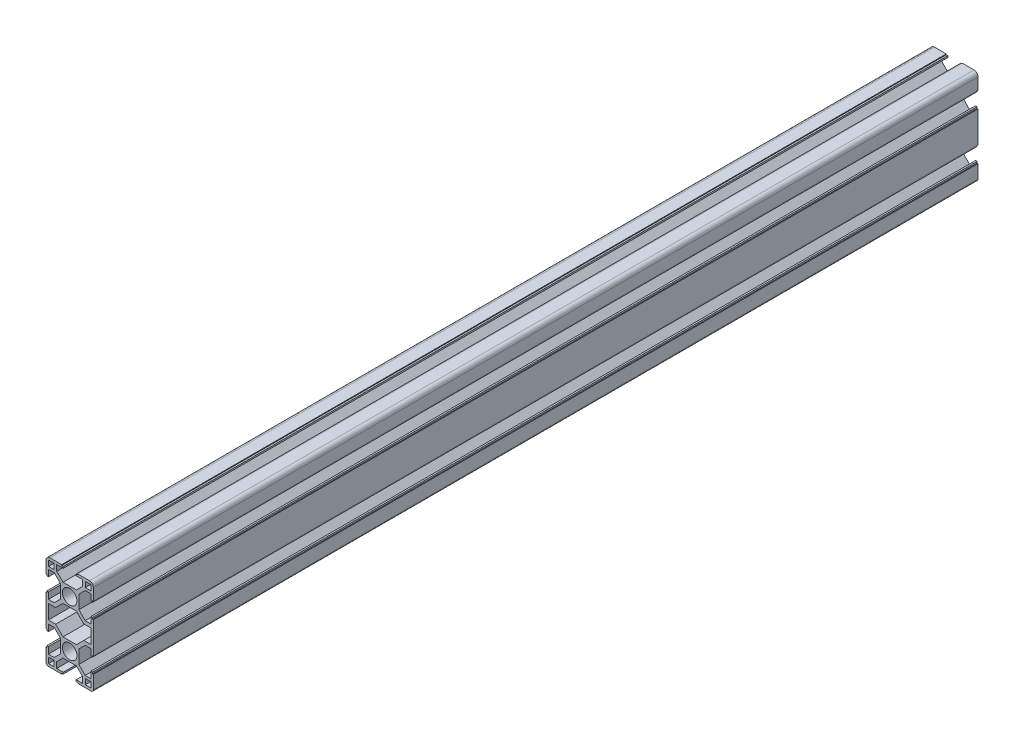
from build123d import *

# Parameters (mm, degrees)
SKETCH1_R                 = 4.6
SKETCH1_W                 = 3.5
SKETCH1_H                 = 3.5
F_30_X_60L_X_R2_5_1_DEPTH = 560
HOLE_WIZARD_1_D           = 6.6
HOLE_WIZARD_1_CBORE_D     = 11
HOLE_WIZARD_1_CBORE_DEPTH = 6.8


with BuildPart() as part:
    # Sketch1 → 铝型材 30 X 60L X R2.5(1) (new body)
    with BuildSketch(Plane(origin=(0, 0, 0), x_dir=(-1, 0, 0), z_dir=(0, 0, -1))):
        with BuildLine():
            Line((-5.1, 15), (-5.1, 14.5))
            Line((-5.1, 14.5), (-4.1, 14.5))
            Line((-4.1, 14.5), (-4.1, 13.5))
            Line((-4.1, 13.5), (-8.25, 13.5))
            Line((-8.25, 13.5), (-8.25, 9.8))
            Line((-8.25, 9.8), (-4.25, 5.8))
            Line((-4.25, 5.8), (4.25, 5.8))
            Line((4.25, 5.8), (8.25, 9.8))
            Line((8.25, 9.8), (8.25, 13.5))
            Line((8.25, 13.5), (4.1, 13.5))
            Line((4.1, 13.5), (4.1, 14.5))
            Line((4.1, 14.5), (5.1, 14.5))
            Line((5.1, 14.5), (5.1, 15))
            Line((5.1, 15), (12.5, 15))
            ThreePointArc((12.5, 15), (14.267766953, 14.267766953), (15, 12.5))
            Line((15, 12.5), (15, 5.1))
            Line((15, 5.1), (14.5, 5.1))
            Line((14.5, 5.1), (14.5, 4.1))
            Line((14.5, 4.1), (13.5, 4.1))
            Line((13.5, 4.1), (13.5, 8.25))
            Line((13.5, 8.25), (9.8, 8.25))
            Line((9.8, 8.25), (5.8, 4.25))
            Line((5.8, 4.25), (5.8, -4.25))
            Line((5.8, -4.25), (9.8, -8.25))
            Line((9.8, -8.25), (13.5, -8.25))
            Line((13.5, -8.25), (13.5, -4.1))
            Line((13.5, -4.1), (14.5, -4.1))
            Line((14.5, -4.1), (14.5, -5.1))
            Line((14.5, -5.1), (15, -5.1))
            Line((15, -5.1), (15, -24.9))
            Line((15, -24.9), (14.5, -24.9))
            Line((14.5, -24.9), (14.5, -25.9))
            Line((14.5, -25.9), (13.5, -25.9))
            Line((13.5, -25.9), (13.5, -21.75))
            Line((13.5, -21.75), (9.8, -21.75))
            Line((9.8, -21.75), (5.8, -25.75))
            Line((5.8, -25.75), (5.8, -34.25))
            Line((5.8, -34.25), (9.8, -38.25))
            Line((9.8, -38.25), (13.5, -38.25))
            Line((13.5, -38.25), (13.5, -34.1))
            Line((13.5, -34.1), (14.5, -34.1))
            Line((14.5, -34.1), (14.5, -35.1))
            Line((14.5, -35.1), (15, -35.1))
            Line((15, -35.1), (15, -43.5))
            ThreePointArc((15, -43.5), (14.560660172, -44.560660172), (13.5, -45))
            Line((13.5, -45), (5.1, -45))
            Line((5.1, -45), (5.1, -44.5))
            Line((5.1, -44.5), (4.1, -44.5))
            Line((4.1, -44.5), (4.1, -43.5))
            Line((4.1, -43.5), (8.25, -43.5))
            Line((8.25, -43.5), (8.25, -39.8))
            Line((8.25, -39.8), (4.25, -35.8))
            Line((4.25, -35.8), (-4.25, -35.8))
            Line((-4.25, -35.8), (-8.25, -39.8))
            Line((-8.25, -39.8), (-8.25, -43.5))
            Line((-8.25, -43.5), (-4.1, -43.5))
            Line((-4.1, -43.5), (-4.1, -44.5))
            Line((-4.1, -44.5), (-5.1, -44.5))
            Line((-5.1, -44.5), (-5.1, -45))
            Line((-5.1, -45), (-13.5, -45))
            ThreePointArc((-13.5, -45), (-14.560660172, -44.560660172), (-15, -43.5))
            Line((-15, -43.5), (-15, -35.1))
            Line((-15, -35.1), (-14.5, -35.1))
            Line((-14.5, -35.1), (-14.5, -34.1))
            Line((-14.5, -34.1), (-13.5, -34.1))
            Line((-13.5, -34.1), (-13.5, -38.25))
            Line((-13.5, -38.25), (-9.8, -38.25))
            Line((-9.8, -38.25), (-5.8, -34.25))
            Line((-5.8, -34.25), (-5.8, -25.75))
            Line((-5.8, -25.75), (-9.8, -21.75))
            Line((-9.8, -21.75), (-13.5, -21.75))
            Line((-13.5, -21.75), (-13.5, -25.9))
            Line((-13.5, -25.9), (-14.5, -25.9))
            Line((-14.5, -25.9), (-14.5, -24.9))
            Line((-14.5, -24.9), (-15, -24.9))
            Line((-15, -24.9), (-15, -5.1))
            Line((-15, -5.1), (-14.5, -5.1))
            Line((-14.5, -5.1), (-14.5, -4.1))
            Line((-14.5, -4.1), (-13.5, -4.1))
            Line((-13.5, -4.1), (-13.5, -8.25))
            Line((-13.5, -8.25), (-9.8, -8.25))
            Line((-9.8, -8.25), (-5.8, -4.25))
            Line((-5.8, -4.25), (-5.8, 4.25))
            Line((-5.8, 4.25), (-9.8, 8.25))
            Line((-9.8, 8.25), (-13.5, 8.25))
            Line((-13.5, 8.25), (-13.5, 4.1))
            Line((-13.5, 4.1), (-14.5, 4.1))
            Line((-14.5, 4.1), (-14.5, 5.1))
            Line((-14.5, 5.1), (-15, 5.1))
            Line((-15, 5.1), (-15, 12.5))
            ThreePointArc((-15, 12.5), (-14.267766953, 14.267766953), (-12.5, 15))
            Line((-12.5, 15), (-5.1, 15))
        make_face()
        Circle(SKETCH1_R, mode=Mode.SUBTRACT)
        with Locations((0, -30)):
            Circle(SKETCH1_R, mode=Mode.SUBTRACT)
        Polygon((8.9, -10.45), (4.25, -5.8), (-4.25, -5.8), (-8.9, -10.45), (-13.5, -10.45), (-13.5, -19.55), (-8.9, -19.55), (-4.25, -24.2), (4.25, -24.2), (8.9, -19.55), (13.5, -19.55), (13.5, -10.45), align=None, mode=Mode.SUBTRACT)
        with Locations((-11.625, 11.625)):
            Rectangle(SKETCH1_W, SKETCH1_H, mode=Mode.SUBTRACT)
        with Locations((11.625, 11.625)):
            Rectangle(SKETCH1_W, SKETCH1_H, mode=Mode.SUBTRACT)
        with Locations((-11.625, -41.625)):
            Rectangle(SKETCH1_W, SKETCH1_H, mode=Mode.SUBTRACT)
        with Locations((11.625, -41.625)):
            Rectangle(SKETCH1_W, SKETCH1_H, mode=Mode.SUBTRACT)
    extrude(amount=F_30_X_60L_X_R2_5_1_DEPTH)

    # 打孔尺寸(%根据)内六角圆柱头螺钉的类型1 (through all)
    with Locations(Plane.ZY.offset(15)):
        with Locations((-550, 0), (-487.5, 0), (-487.5, -30), (-550, -30), (-520, -30), (-520, 0)):
            CounterBoreHole(HOLE_WIZARD_1_D / 2, HOLE_WIZARD_1_CBORE_D / 2, HOLE_WIZARD_1_CBORE_DEPTH)


solid = part.part
